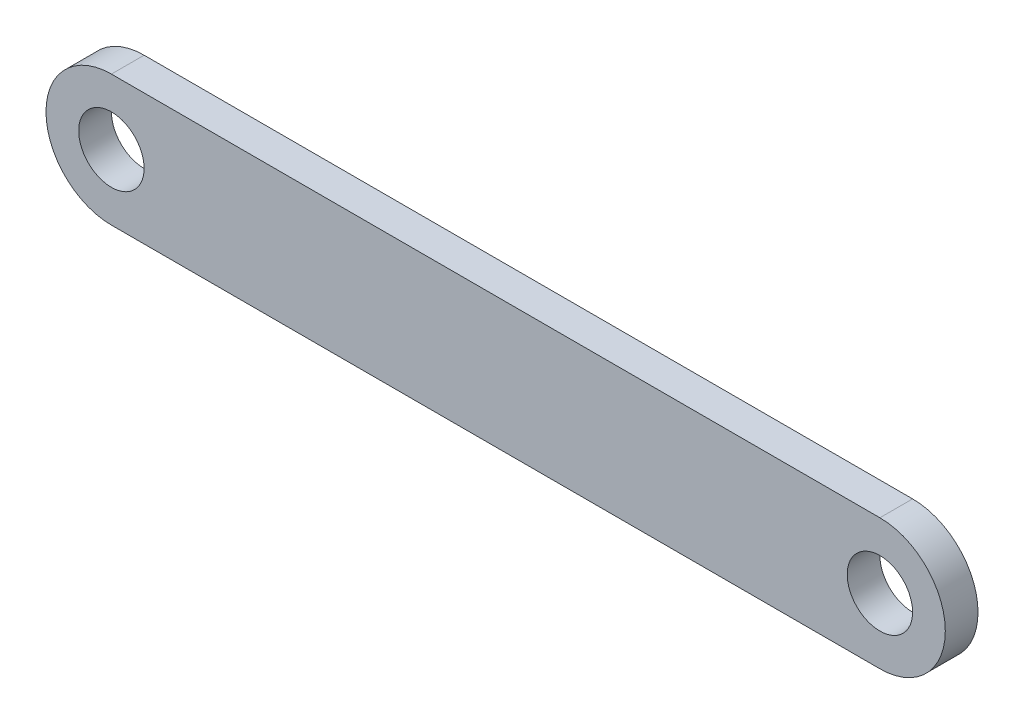
SolidWorks part; units mm, degrees
ref_plane "Front Plane" through (0, 0, 0) normal (0, 0, 1) x (1, 0, 0)
ref_plane "Top Plane" through (0, 0, 0) normal (0, 1, 0) x (1, 0, 0)
ref_plane "Right Plane" through (0, 0, 0) normal (1, 0, 0) x (0, 0, -1)
sketch "Sketch1" plane through (0, 0, 0) normal (0, 0, 1) x (1, 0, 0)
  line L0 (-117.5, 0) -> (117.5, 0) construction
  line L1 (-117.5, 20) -> (117.5, 20)
  line L2 (-117.5, -20) -> (117.5, -20)
  arc A0 (-117.5, 20) -> (-117.5, -20) centre (-117.5, 0) ccw
  arc A1 (117.5, -20) -> (117.5, 20) centre (117.5, 0) ccw
  point P2 (0, 0)
  dimension "D1" = 20
  dimension "D2" = 235
extrude "Boss-Extrude1" add sketch "Sketch1" along normal blind 10
sketch "Sketch2" plane through (0, 0, 10) normal (0, 0, 1) x (1, 0, 0)
  circle A0 centre (-117.5, 0) radius 10
  circle A1 centre (117.5, 0) radius 10
  dimension "D1" = 20
extrude "Cut-Extrude1" cut sketch "Sketch2" against normal through all
